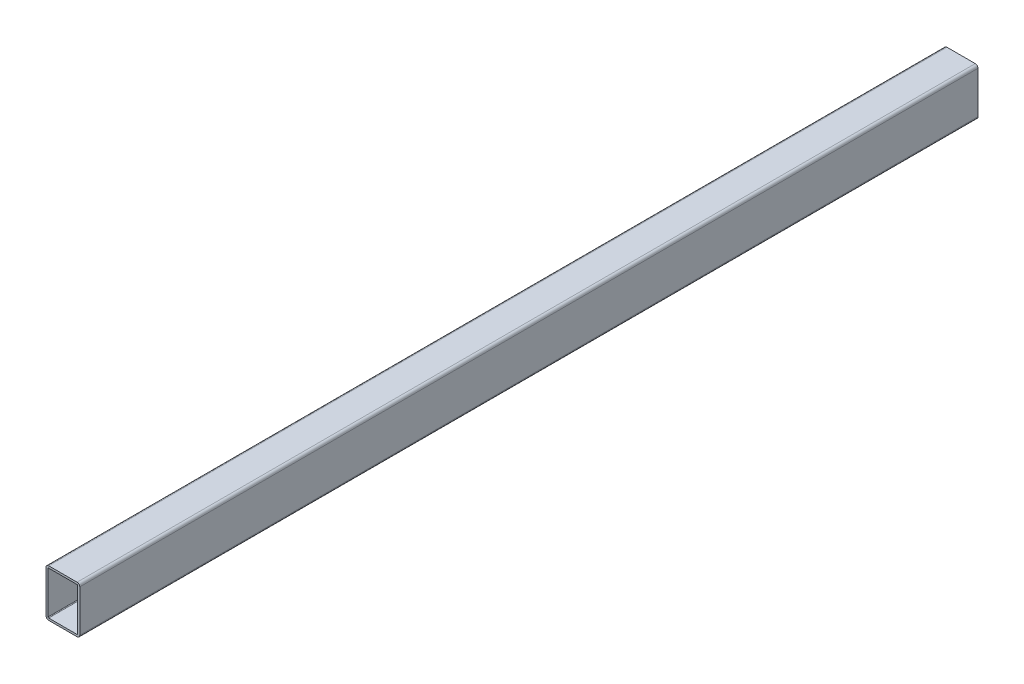
from build123d import *

# Parameters (mm, degrees)
EXTRUDE_THIN1_DEPTH = 1330


with BuildPart() as part:
    # Sketch1 → Extrude-Thin1 (new body)
    with BuildSketch(Plane.XY):
        with BuildLine():
            Line((-25, 31), (-25, -31))
            ThreePointArc((-25, -31), (-23.828427125, -33.828427125), (-21, -35))
            Line((-21, -35), (21, -35))
            ThreePointArc((21, -35), (23.828427125, -33.828427125), (25, -31))
            Line((25, -31), (25, 31))
            ThreePointArc((25, 31), (23.828427125, 33.828427125), (21, 35))
            Line((21, 35), (-21, 35))
            ThreePointArc((-21, 35), (-23.828427125, 33.828427125), (-25, 31))
        make_face()
        with BuildLine():
            Line((-22, 31), (-22, -31))
            ThreePointArc((-22, -31), (-21.707106781, -31.707106781), (-21, -32))
            Line((-21, -32), (21, -32))
            ThreePointArc((21, -32), (21.707106781, -31.707106781), (22, -31))
            Line((22, -31), (22, 31))
            ThreePointArc((22, 31), (21.707106781, 31.707106781), (21, 32))
            Line((21, 32), (-21, 32))
            ThreePointArc((-21, 32), (-21.707106781, 31.707106781), (-22, 31))
        make_face(mode=Mode.SUBTRACT)
    extrude(amount=EXTRUDE_THIN1_DEPTH)


solid = part.part
